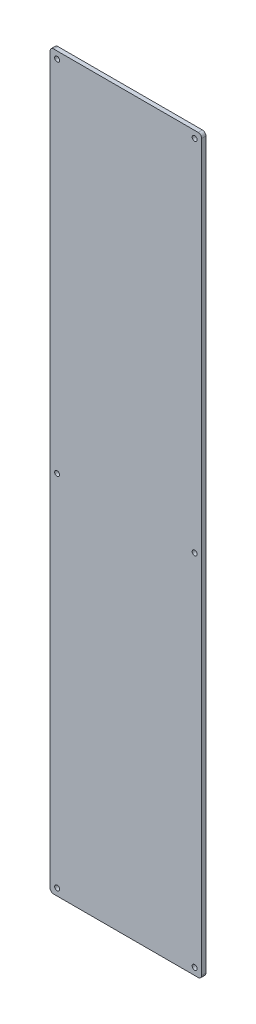
from build123d import *

# Parameters (mm, degrees)
SKETCH_1_W            = 215
SKETCH_1_H            = 1038
EXTRUDE_1_DEPTH       = 6
HOLE_WIZARD_7_0_7_1_D = 7
FILLET_1_R            = 5


with BuildPart() as part:
    # 草图1 → 凸台-拉伸1 (new body)
    with BuildSketch(Plane.XY):
        Rectangle(SKETCH_1_W, SKETCH_1_H)
    extrude(amount=EXTRUDE_1_DEPTH)

    # Ø7.0 (7) 直径孔1 (through all)
    with Locations(Plane(origin=(0, 0, 0), x_dir=(-1, 0, 0), z_dir=(0, 0, -1))):
        with Locations((-97.5, 509), (-97.5, -509), (97.5, 509), (97.5, -509), (-97.5, 0), (97.5, 0)):
            Hole(HOLE_WIZARD_7_0_7_1_D / 2)

    # 圆角1
    fillet_1_edges = [part.edges().sort_by_distance(p)[0] for p in [
        (107.5, -519, 3),
        (-107.5, -519, 3),
        (-107.5, 519, 3),
        (107.5, 519, 3),
    ]]
    fillet(fillet_1_edges, radius=FILLET_1_R)


solid = part.part
